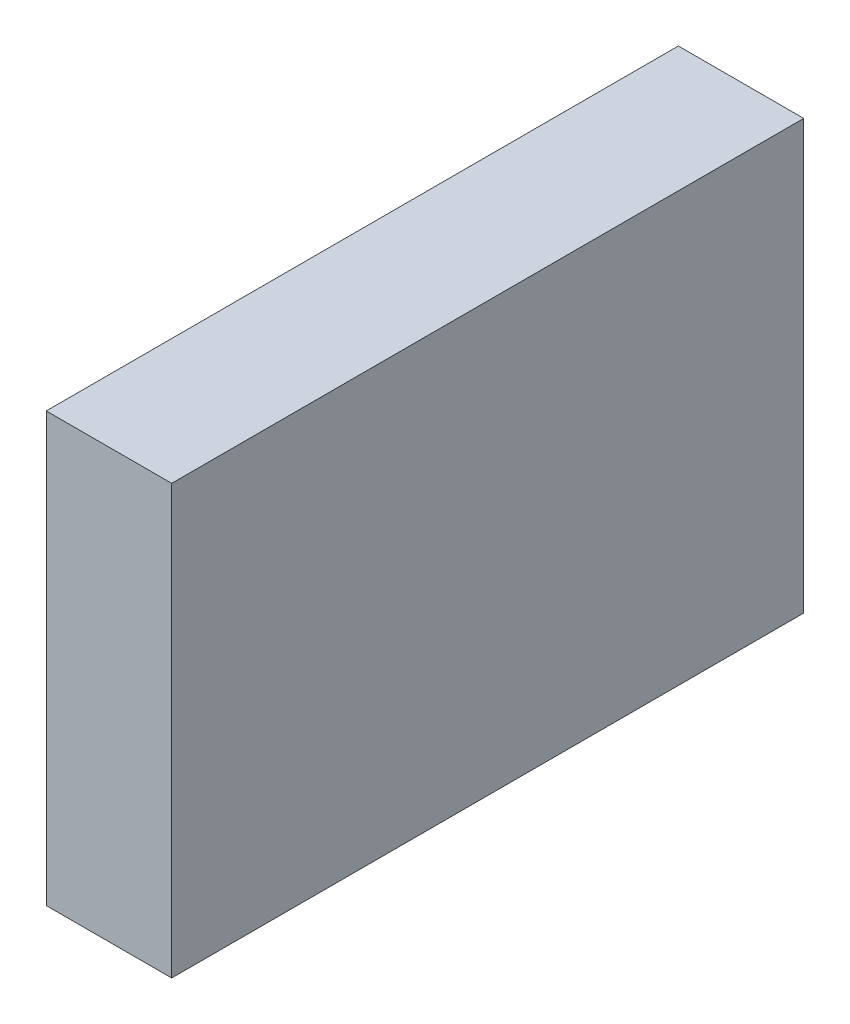
SolidWorks part; units mm, degrees
material "Q345B"
ref_plane "Front Plane" through (0, 0, 0) normal (0, 0, 1) x (1, 0, 0)
ref_plane "Top Plane" through (0, 0, 0) normal (0, 1, 0) x (1, 0, 0)
ref_plane "Right Plane" through (0, 0, 0) normal (1, 0, 0) x (0, 0, -1)
sketch "Sketch2" plane through (0, 0, 0) normal (0, 1, 0) x (1, 0, 0)
  line L0 (-131.395, 0) -> (113.7022, 0) construction
  line L1 (0, 164.1787) -> (0, -121.5078) construction
  line L3 (-12.5, 63) -> (12.5, 63)
  line L4 (-12.5, 63) -> (-12.5, -63)
  line L5 (-12.5, -63) -> (12.5, -63)
  line L6 (12.5, 63) -> (12.5, -63)
  dimension "D1" = 126
  dimension "D2" = 25
  dimension "D3" = 12.5
extrude "Boss-Extrude1" add sketch "Sketch2" along normal mid plane 85.4
